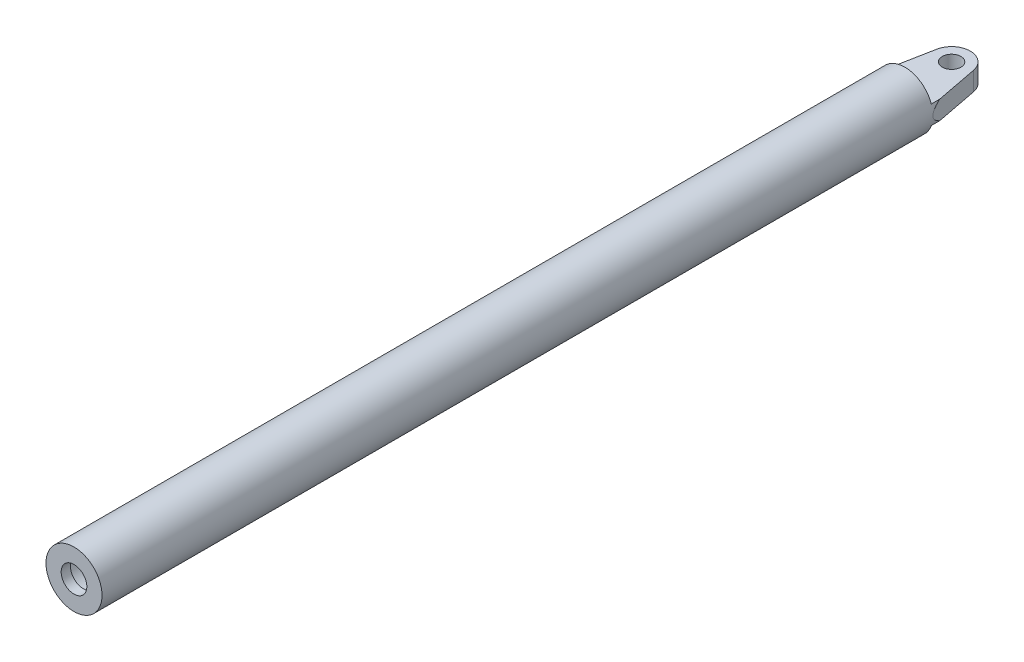
from build123d import *
from build123d.topology import SkipClean

# Parameters (mm, degrees)
SKETCH_1_R          = 60
SKETCH_1_R_2        = 45
EXTRUDE_1_DEPTH     = 1780
SKETCH_2_R          = 20
EXTRUDE_2_DEPTH     = 20
SKETCH_3_R          = 50
EXTRUDE_3_DEPTH     = 40
SKETCH_4_OUTSIDE_W  = 507.498
SKETCH_4_OUTSIDE_H  = 507.498
SKETCH_4_OUTSIDE_R  = 60
CUT_EXTRUDE_1_DEPTH = 1783.021324227
EXTRUDE_START       = -20
SKETCH_5_R          = 60
SKETCH_5_R_2        = 27.5
EXTRUDE_4_DEPTH     = 20


with BuildPart() as part:
    # 草图1 → 凸台-拉伸1 (new body)
    with BuildSketch(Plane.XY):
        Circle(SKETCH_1_R)
        Circle(SKETCH_1_R_2, mode=Mode.SUBTRACT)
    extrude(amount=EXTRUDE_1_DEPTH)

    # 草图2 → 凸台-拉伸2 (add, symmetric)
    with BuildSketch(Plane(origin=(0, 0, 0), x_dir=(1, 0, 0), z_dir=(0, 1, 0))):
        with BuildLine():
            Line((-60, 0), (-39.2777975, 107.5666785))
            ThreePointArc((-39.2777975, 107.5666785), (0, 140), (39.2777975, 107.5666785))
            Line((39.2777975, 107.5666785), (60, 0))
            Line((60, 0), (-60, 0))
        make_face()
        with Locations(Location((0, 100, 0), (0, 0, 270))):
            Circle(SKETCH_2_R, mode=Mode.SUBTRACT)
    extrude(amount=EXTRUDE_2_DEPTH, both=True)

    # 草图3 → 凸台-拉伸3 (add)
    with BuildSketch(Plane(origin=(0, 0, 0), x_dir=(-1, 0, 0), z_dir=(0, 0, -1))):
        Circle(SKETCH_3_R)
    extrude(amount=-EXTRUDE_3_DEPTH)

    # 草图4 outside → 切除-拉伸1 (cut, through all)
    with BuildSketch(Plane(origin=(0, 0, 0), x_dir=(-1, 0, 0), z_dir=(0, 0, -1))):
        Rectangle(SKETCH_4_OUTSIDE_W, SKETCH_4_OUTSIDE_H)
        with Locations(Location((0, 0, 0), (0, 0, 19.471220634))):
            Circle(SKETCH_4_OUTSIDE_R, mode=Mode.SUBTRACT)
    extrude(amount=CUT_EXTRUDE_1_DEPTH, mode=Mode.SUBTRACT)

    # 草图5 → 凸台-拉伸4 (add)
    with SkipClean():  # the faces are left unmerged after this step: merging them gives an invalid solid
        with BuildSketch(Plane.XY.offset(1780).offset(EXTRUDE_START)):
            with Locations(Location((0, 0, 0), (0, 0, 160.528779366))):
                Circle(SKETCH_5_R)
            Circle(SKETCH_5_R_2, mode=Mode.SUBTRACT)
        extrude(amount=EXTRUDE_4_DEPTH)


solid = part.part
